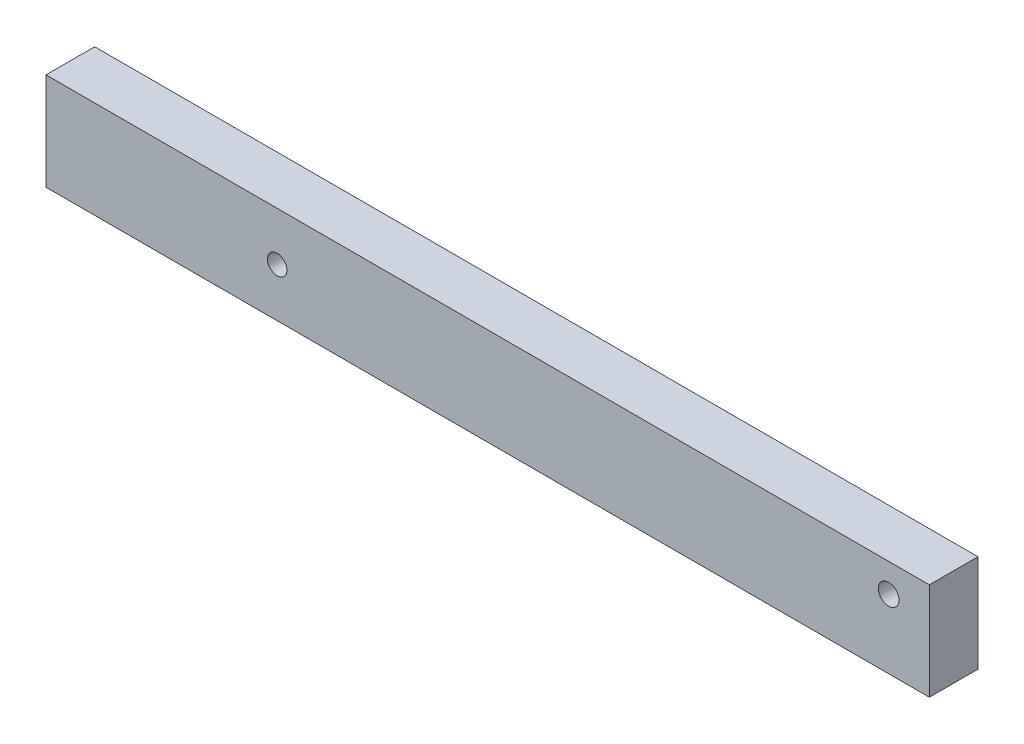
from build123d import *

# Parameters (mm, degrees)
SKETCH_2_W          = 400
SKETCH_2_H          = 40
SKETCH_2_R          = 4
EXTRUDE_1_DEPTH     = 20
SKETCH_4_W          = 20
SKETCH_4_H          = 40
EXTRUDE_2_DEPTH     = 248
HOLE_WIZARD_M10_1_D = 8.5
SKETCH_9_W          = 20
SKETCH_9_H          = 40
CUT_EXTRUDE_2_DEPTH = 285


with BuildPart() as part:
    # 草图2 → 凸台-拉伸1 (new body)
    with BuildSketch(Plane.XY):
        Rectangle(SKETCH_2_W, SKETCH_2_H)
        with Locations((180, 0)):
            Circle(SKETCH_2_R, mode=Mode.SUBTRACT)
    extrude(amount=EXTRUDE_1_DEPTH)

    # 草图4 → 凸台-拉伸2 (add)
    with BuildSketch(Plane(origin=(200, 0, 0), x_dir=(0, 0, -1), z_dir=(1, 0, 0))):
        with Locations((-10, 0)):
            Rectangle(SKETCH_4_W, SKETCH_4_H)
    extrude(amount=EXTRUDE_2_DEPTH)

    # M10 螺纹孔1 (through all)
    with Locations(Plane.XY.offset(20)):
        with Locations((431.276, 8.288)):
            Hole(HOLE_WIZARD_M10_1_D / 2)

    # 草图9 → 切除-拉伸2 (cut)
    with BuildSketch(Plane.ZY.offset(200)):
        with Locations((10, 0)):
            Rectangle(SKETCH_9_W, SKETCH_9_H)
    extrude(amount=-CUT_EXTRUDE_2_DEPTH, mode=Mode.SUBTRACT)


solid = part.part
